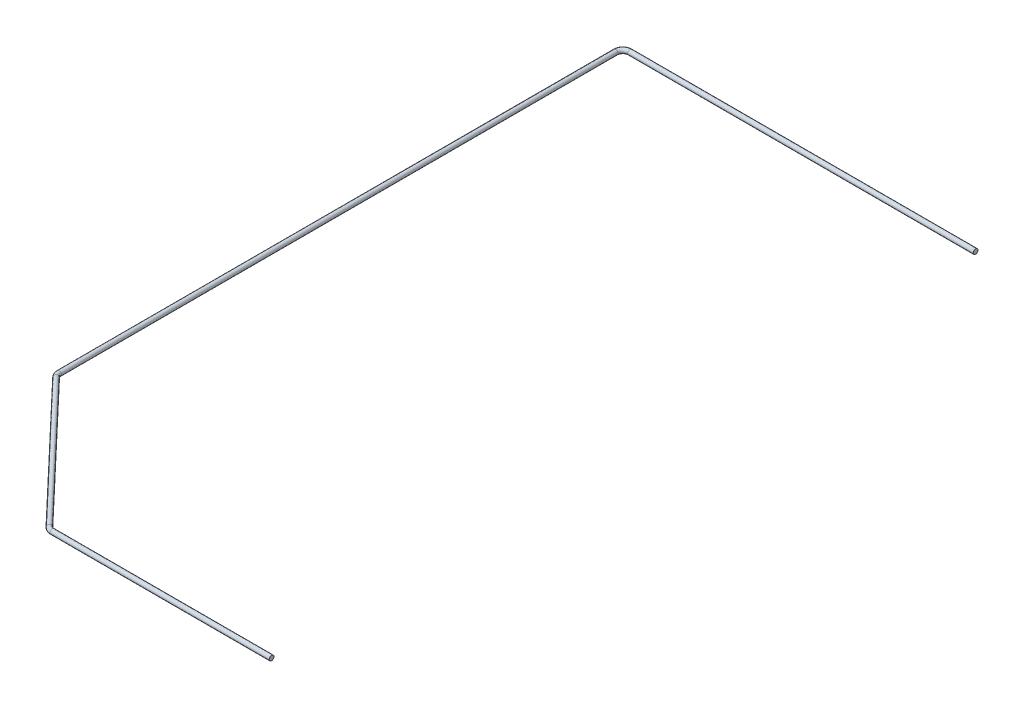
from build123d import *

# Parameters (mm, degrees)
SKETCH2_R = 3


with BuildPart() as part:
    # Sweep1: sweep along a path in Sketch1
    with BuildLine(Plane(origin=(0, 0, 0), x_dir=(1, 0, 0), z_dir=(0, 1, 0))) as sweep1_path:
        Line((0, 0), (-432.5, 0))
        ThreePointArc((-432.5, 0), (-438.863961031, -2.636038969), (-441.5, -9))
        Line((-441.5, -9), (-441.5, -705.408118144))
        ThreePointArc((-441.5, -705.408118144), (-440.858887638, -708.744133349), (-439.026889456, -711.604868424))
        Line((-439.026889456, -711.604868424), (-280.861457438, -878.19675028))
        ThreePointArc((-280.861457438, -878.19675028), (-277.886275141, -880.269545106), (-274.334567982, -881))
        Line((-274.334567982, -881), (0, -881))
    # Sketch2 → Sweep1 (sweep)
    with BuildSketch(Plane(origin=(0, 0, 0), x_dir=(0, 0, -1), z_dir=(1, 0, 0))):
        Circle(SKETCH2_R)
    sweep(path=sweep1_path.line)


solid = part.part
